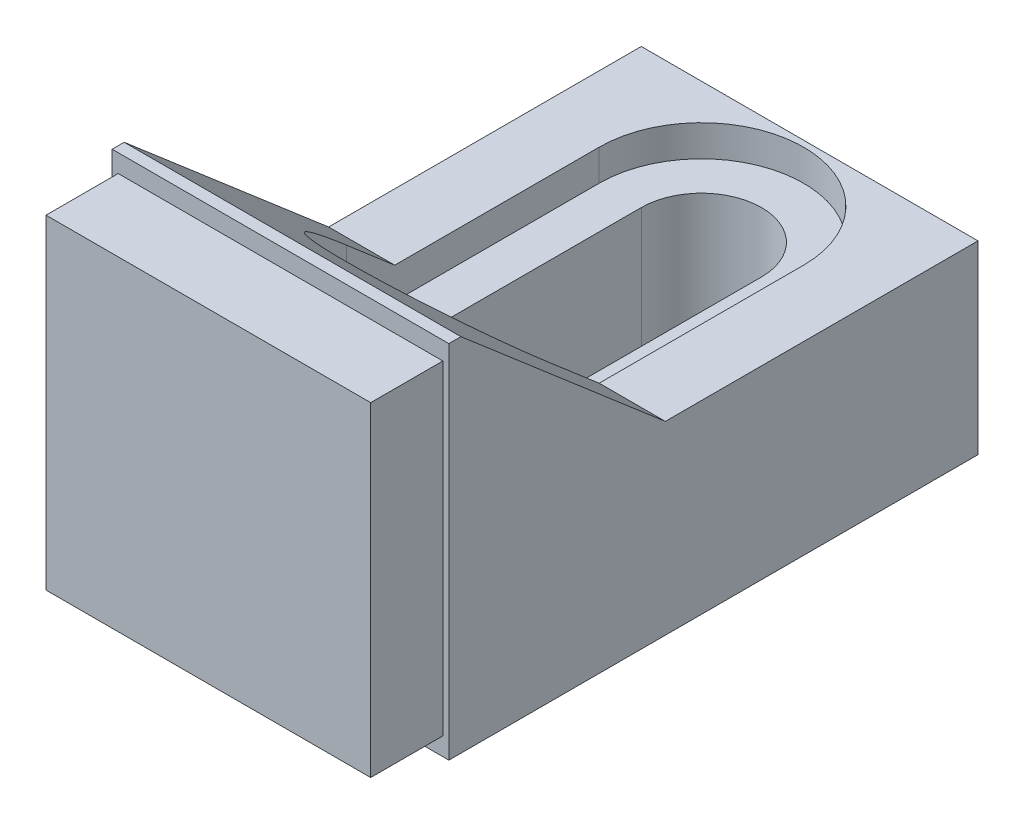
from build123d import *

# Parameters (mm, degrees)
SKETCH1_W               = 13.5
SKETCH1_H               = 13.5
BOSS_EXTRUDE1_DEPTH     = 1.5
SKETCH2_W               = 14
SKETCH2_H               = 15
BOSS_EXTRUDE2_DEPTH     = 22
CUT_EXTRUDE2_DEPTH      = 29.363709207
CUT_EXTRUDE2_DEPTH_BACK = 29.363709207
CUT_EXTRUDE3_DEPTH      = 8.6
CUT_EXTRUDE4_DEPTH      = 11.3


with BuildPart() as part:
    # Sketch1 → Boss-Extrude1 (new, symmetric)
    with BuildSketch(Plane.XY):
        Rectangle(SKETCH1_W, SKETCH1_H)
    extrude(amount=BOSS_EXTRUDE1_DEPTH, both=True)

    # Sketch2 → Boss-Extrude2 (add)
    with BuildSketch(Plane(origin=(0, 0, -1.5), x_dir=(-1, 0, 0), z_dir=(0, 0, -1))):
        Rectangle(SKETCH2_W, SKETCH2_H)
    extrude(amount=BOSS_EXTRUDE2_DEPTH)

    # Sketch3 → Cut-Extrude2 (cut, two sides: drawn at the far end of the back side and taken through both)
    with BuildSketch(Plane(origin=(7, 0, 0), x_dir=(0, 0, -1), z_dir=(1, 0, 0)).offset(-CUT_EXTRUDE2_DEPTH_BACK)):
        Polygon((85.930906916, 0.2), (23.5, 0.2), (10.5, 0.2), (2, 7.5), (-45.361724521, 48.175363412), (-2.507621852, 165.452805564), (128.785009585, 117.477442152), align=None)
    extrude(amount=CUT_EXTRUDE2_DEPTH + CUT_EXTRUDE2_DEPTH_BACK, mode=Mode.SUBTRACT)

    # Sketch5 → Cut-Extrude3 (cut)
    with BuildSketch(Plane(origin=(0, 7.5, 0), x_dir=(1, 0, 0), z_dir=(0, 1, 0))):
        with BuildLine():
            Line((-4.25, 19), (-4.25, 8.5))
            ThreePointArc((-4.25, 8.5), (0, 4.25), (4.25, 8.5))
            Line((4.25, 8.5), (4.25, 19))
            ThreePointArc((4.25, 19), (0, 23.25), (-4.25, 19))
        make_face()
    extrude(amount=-CUT_EXTRUDE3_DEPTH, mode=Mode.SUBTRACT)

    # Sketch4 → Cut-Extrude4 (cut)
    with BuildSketch(Plane(origin=(0, 0.2, 0), x_dir=(1, 0, 0), z_dir=(0, 1, 0))):
        with BuildLine():
            Line((2.5, 19), (2.5, 8.5))
            ThreePointArc((2.5, 8.5), (0, 6), (-2.5, 8.5))
            Line((-2.5, 8.5), (-2.5, 19))
            ThreePointArc((-2.5, 19), (0, 21.5), (2.5, 19))
        make_face()
    extrude(amount=-CUT_EXTRUDE4_DEPTH, mode=Mode.SUBTRACT)


solid = part.part
